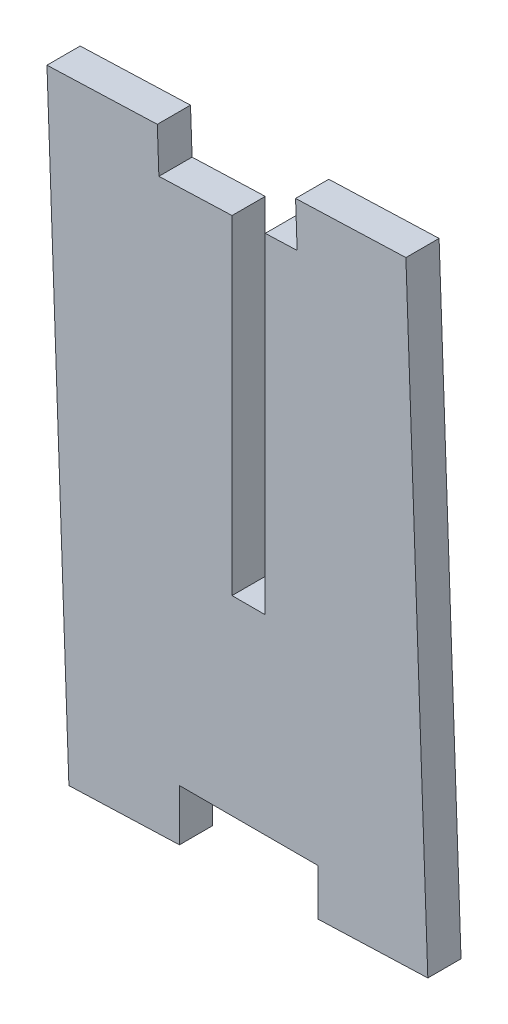
SolidWorks part; units mm, degrees
material "Q235B"
ref_plane "Front Plane" through (0, 0, 0) normal (0, 0, 1) x (1, 0, 0)
ref_plane "Top Plane" through (0, 0, 0) normal (0, 1, 0) x (1, 0, 0)
ref_plane "Right Plane" through (0, 0, 0) normal (1, 0, 0) x (0, 0, -1)
sketch "Sketch1" plane through (0, 0, 0) normal (0, 0, 1) x (1, 0, 0)
  line L0 (135.3024, 83.362) -> (139.5037, -34.009) construction
  line L1 (167.7656, 84.524) -> (98.1537, 84.524) construction
  line L2 (106.5516, -20.5639) -> (102.587, 90.1961)
  line L3 (106.5516, -20.5639) -> (126.5284, -19.8488)
  line L4 (126.5284, -19.8488) -> (126.5284, -10.5639)
  line L5 (151.5292, -18.9539) -> (171.4101, -18.2423)
  line L6 (122.8104, 82.9149) -> (122.5242, 90.9097)
  line L7 (171.4101, -18.2423) -> (167.4455, 92.5177)
  line L8 (147.7944, 83.8092) -> (122.8104, 82.9149)
  line L9 (126.5284, -10.5639) -> (151.5292, -10.5639)
  line L10 (151.5292, -10.5639) -> (151.5292, -18.9539)
  line L11 (122.5242, 90.9097) -> (102.587, 90.1961)
  line L12 (147.7944, 83.8092) -> (147.5082, 91.804)
  line L13 (147.5082, 91.804) -> (167.4455, 92.5177)
  dimension "D1" = 2.05
  dimension "D2" = 90
  dimension "D3" = 8
  dimension "D4" = 110.76
  dimension "D5" = 9.2849
  dimension "D6" = 12.5
  dimension "D7" = 90
  dimension "D8" = 64.9
extrude "Boss-Extrude1" add sketch "Sketch1" along normal blind 6
sketch "Sketch2" plane through (0, 0, 6) normal (0, 0, 1) x (1, 0, 0)
  line L0 (136.0288, 23.9104) -> (142.0288, 23.9104)
  line L2 (136.0288, 83.8856) -> (136.0288, 23.9104)
  line L3 (142.0288, 83.8856) -> (142.0288, 23.9104)
  line L4 (136.0288, 83.8856) -> (142.0288, 83.8856)
  line L8 (126.5284, -10.5639) -> (151.5292, -10.5639) construction
  point P3 (139.0288, -10.5639)
  point P8 (139.0288, 23.9104)
  dimension "D1" = 6
extrude "Cut-Extrude1" cut sketch "Sketch2" against normal blind 6
